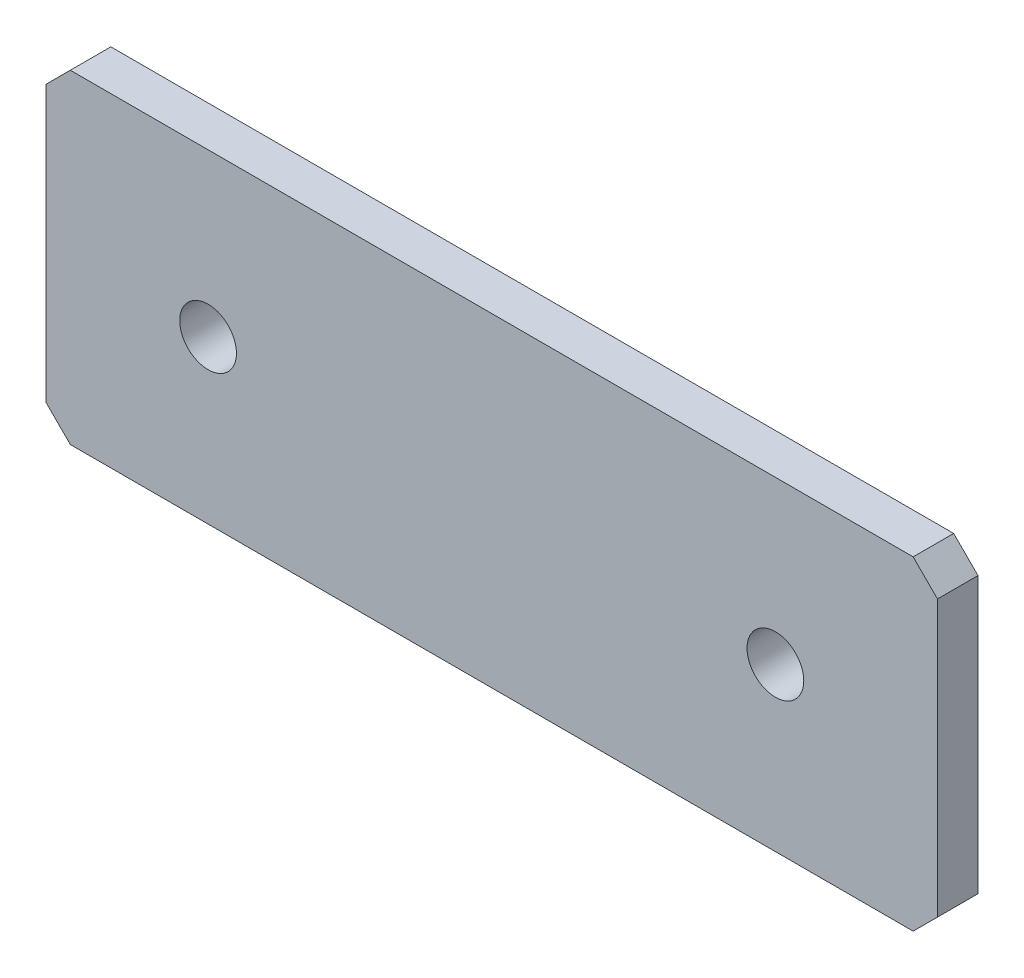
from build123d import *

# Parameters (mm, degrees)
SKETCH1_W           = 110
SKETCH1_H           = 40
SKETCH1_R           = 3.5
BOSS_EXTRUDE1_DEPTH = 5
CHAMFER1_SIZE       = 3


with BuildPart() as part:
    # Sketch1 → Boss-Extrude1 (new body)
    with BuildSketch(Plane.XY):
        Rectangle(SKETCH1_W, SKETCH1_H)
        with Locations((-35, 0)):
            Circle(SKETCH1_R, mode=Mode.SUBTRACT)
        with Locations((35, 0)):
            Circle(SKETCH1_R, mode=Mode.SUBTRACT)
    extrude(amount=BOSS_EXTRUDE1_DEPTH)

    # Chamfer1
    chamfer1_edges = [part.edges().sort_by_distance(p)[0] for p in [
        (55, -20, 2.5),
        (55, 20, 2.5),
        (-55, 20, 2.5),
        (-55, -20, 2.5),
    ]]
    chamfer(chamfer1_edges, length=CHAMFER1_SIZE)


solid = part.part
